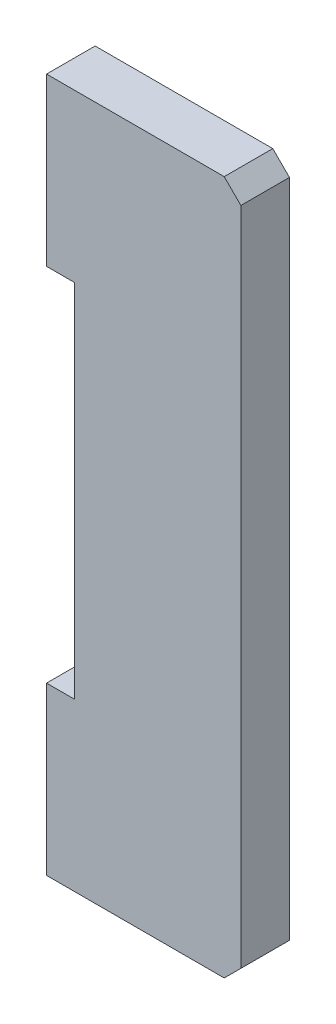
SolidWorks part; units mm, degrees
ref_plane "前视基准面" through (0, 0, 0) normal (0, 0, 1) x (1, 0, 0)
ref_plane "上视基准面" through (0, 0, 0) normal (0, 1, 0) x (1, 0, 0)
ref_plane "右视基准面" through (0, 0, 0) normal (1, 0, 0) x (0, 0, -1)
sketch "草图1" plane through (0, 0, 0) normal (0, 0, 1) x (1, 0, 0)
  line L0 (-140, 0) -> (0, 0)
  line L4 (-120, -120) -> (-120, -380)
  line L7 (-120, -120) -> (-140, -120)
  line L8 (-140, 0) -> (-140, -120)
  line L11 (-120, -380) -> (-140, -380)
  line L12 (-140, -500) -> (-140, -380)
  line L13 (0, 0) -> (0, -500)
  line L14 (0, -500) -> (-140, -500)
  line L15 (-140, 30) -> (-140, -120) construction
  line L17 (-140, -530) -> (-140, -380) construction
  dimension "D1" = 120
  dimension "D2" = 120
  dimension "D3" = 120
  dimension "D4" = 500
extrude "凸台-拉伸1" add sketch "草图1" along normal blind 35
chamfer "倒角1" distance 12 angle 45 2 edges at (0, -500, 17.5) (0, 0, 17.5)
